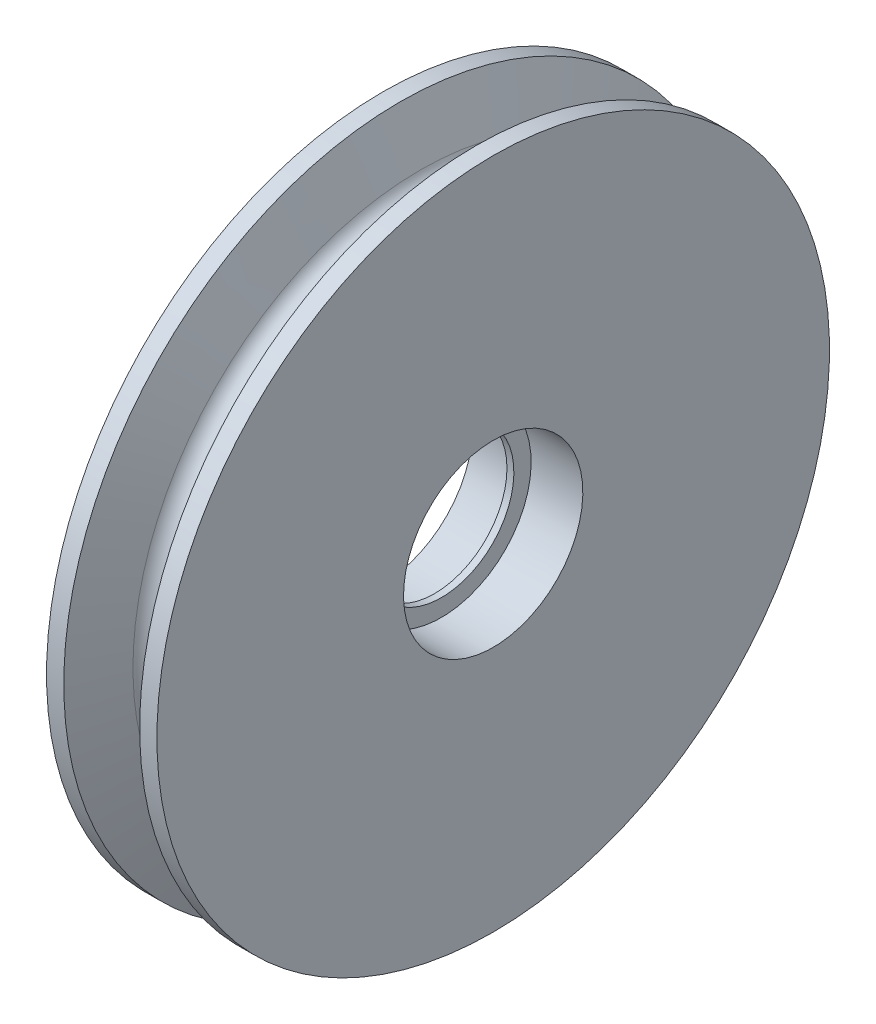
SolidWorks part; units mm, degrees
material "Q235B"
ref_plane "Front Plane" through (0, 0, 0) normal (0, 0, 1) x (1, 0, 0)
ref_plane "Top Plane" through (0, 0, 0) normal (0, 1, 0) x (1, 0, 0)
ref_plane "Right Plane" through (0, 0, 0) normal (1, 0, 0) x (0, 0, -1)
sketch "Sketch1" plane through (0, 0, 0) normal (0, 0, 1) x (1, 0, 0)
  line L0 (-16, 0) -> (-16, 97.5)
  line L1 (-16, 97.5) -> (-11, 97.5)
  line L2 (-11, 97.5) -> (-5.0716, 83.3719)
  line L3 (0, 82.4776) -> (0, 0) construction
  line L4 (0, 0) -> (-16, 0) construction
  line L5 (11, 97.5) -> (5.0716, 83.3719)
  line L6 (16, 97.5) -> (11, 97.5)
  line L7 (16, 0) -> (16, 97.5)
  line L8 (16, 0) -> (-16, 0)
  arc A0 (-5.0716, 83.3719) -> (5.0716, 83.3719) centre (0, 85.5) ccw
  dimension "D1" = 195
  dimension "D3" = 5.5
  dimension "D2" = 171
  dimension "D4" = 32
  dimension "D5" = 5
revolve "Revolve1" add sketch "Sketch1" angle 360 about L8
sketch "Sketch2" plane through (16, 0, 0) normal (1, 0, 0) x (0, 0, -1)
  circle A0 centre (0, 0) radius 21
  dimension "D1" = 42
extrude "Cut-Extrude1" cut sketch "Sketch2" against normal up to next
sketch "Sketch3" plane through (16, 0, 0) normal (1, 0, 0) x (0, 0, -1)
  circle A0 centre (0, 0) radius 26
  dimension "D1" = 52
extrude "Cut-Extrude2" cut sketch "Sketch3" against normal blind 15
mirror "Mirror1" about plane through (0, 0, 0) normal (1, 0, 0) of "Cut-Extrude2"
